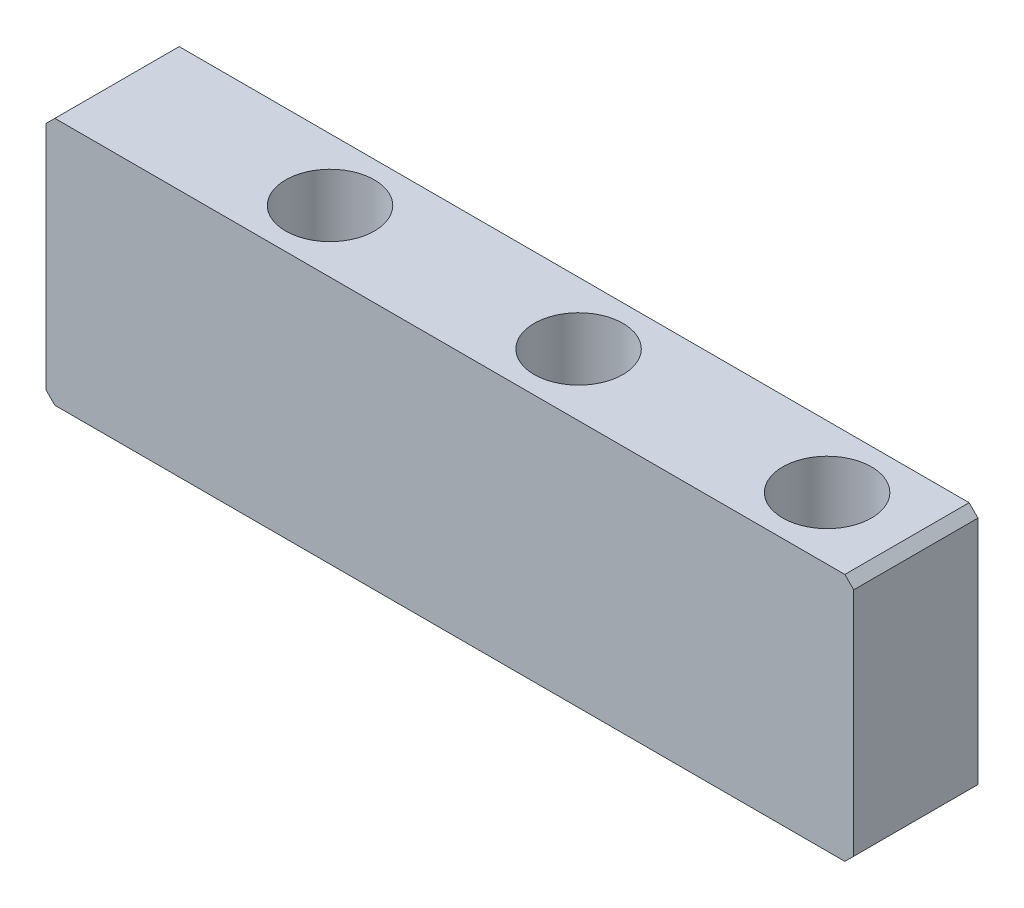
from build123d import *

# Parameters (mm, degrees)
SKETCH1_W                                            = 91
SKETCH1_H                                            = 28
BOSS_EXTRUDE1_DEPTH                                  = 7
M6_TAPPED_HOLE1_D                                    = 5
M6_TAPPED_HOLE1_DEPTH                                = 15
M6_TAPPED_HOLE1_TIP                                  = 1.502151548
HOLE_SIZE_PER_SOCKET_HEAD_CAP_SCREW_TYPE_D           = 5.5
HOLE_SIZE_PER_SOCKET_HEAD_CAP_SCREW_TYPE_CBORE_D     = 10
HOLE_SIZE_PER_SOCKET_HEAD_CAP_SCREW_TYPE_CBORE_DEPTH = 10
CHAMFER1_SIZE                                        = 1


with BuildPart() as part:
    # Sketch1 → Boss-Extrude1 (new, symmetric)
    with BuildSketch(Plane.XY):
        Rectangle(SKETCH1_W, SKETCH1_H)
    extrude(amount=BOSS_EXTRUDE1_DEPTH, both=True)

    # M6 Tapped Hole1
    with Locations(Plane.ZY.offset(45.5)):
        with Locations((0, -7), (0, 7)):
            Hole(M6_TAPPED_HOLE1_D / 2, depth=M6_TAPPED_HOLE1_DEPTH)
            with Locations((0, 0, -(M6_TAPPED_HOLE1_DEPTH + M6_TAPPED_HOLE1_TIP / 2))):  # 118° drill point
                Cone(0, M6_TAPPED_HOLE1_D / 2, M6_TAPPED_HOLE1_TIP, mode=Mode.SUBTRACT)

    # Hole Size per Socket Head Cap Screw Type1 (through all)
    with Locations(Plane(origin=(0, 14, 0), x_dir=(1, 0, 0), z_dir=(0, 1, 0))):
        with Locations((7.5, 0), (-20.5, 0), (35.5, 0)):
            CounterBoreHole(HOLE_SIZE_PER_SOCKET_HEAD_CAP_SCREW_TYPE_D / 2, HOLE_SIZE_PER_SOCKET_HEAD_CAP_SCREW_TYPE_CBORE_D / 2, HOLE_SIZE_PER_SOCKET_HEAD_CAP_SCREW_TYPE_CBORE_DEPTH)

    # Chamfer1
    chamfer1_edges = [part.edges().sort_by_distance(p)[0] for p in [
        (45.5, -14, 0),
        (-45.5, -14, 0),
        (-45.5, 14, 0),
        (45.5, 14, 0),
    ]]
    chamfer(chamfer1_edges, length=CHAMFER1_SIZE)


solid = part.part
